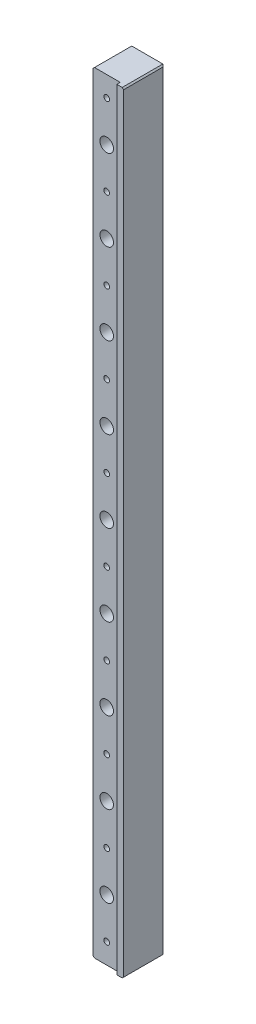
SolidWorks part; units mm, degrees
material "Q235-A"
ref_plane "Front/Back" through (0, 0, 0) normal (0, 0, 1) x (1, 0, 0)
ref_plane "Top/Bottom" through (0, 0, 0) normal (0, 1, 0) x (1, 0, 0)
ref_plane "Right/Left" through (0, 0, 0) normal (1, 0, 0) x (0, 0, -1)
sketch "Sketch1" plane through (0, 0, 0) normal (0, 0, 1) x (1, 0, 0)
  line L0 (-12.5, -285) -> (12.5, 285) construction
  line L1 (-12.5, 285) -> (12.5, 285)
  line L2 (-12.5, 285) -> (-12.5, -285)
  line L3 (-12.5, -285) -> (12.5, -285)
  line L4 (12.5, 285) -> (12.5, -285)
  point P4 (0, 0)
  dimension "D1" = 25
  dimension "D2" = 570
extrude "Extrude1" add sketch "Sketch1" along normal mid plane 30
chamfer "Chamfer1" distance 1 angle 45 4 edges at (12.5, 285, 0) (-12.5, 285, 0) (12.5, -285, 0) (-12.5, -285, 0)
sketch "草图1" plane through (0, 0, 15) normal (0, 0, 1) x (1, 0, 0)
  line L0 (-11.5, -285) -> (11.5, -285) construction
  line L3 (-12.5, 285) -> (7.5, 285)
  line L6 (0, 285) -> (0, -286.2731) construction
  line L7 (11.5, 285) -> (-11.5, 285) construction
  line L9 (-12.5, 285) -> (-12.5, -285)
  line L10 (-12.5, -285) -> (7.5, -285)
  line L11 (7.5, 285) -> (7.5, -285)
  line L12 (12.5, -284) -> (12.5, 284) construction
  line L13 (11.5, 285) -> (-11.5, 285) construction
  line L14 (-12.5, 284) -> (-12.5, -284) construction
  dimension "D1" = 5
extrude "Cut-Extrude1" cut sketch "草图1" against normal blind 2.5
chamfer "Chamfer2" distance 1 angle 45 2 edges at (12.5, 0, -15) (-12.5, 0, -15)
hole_wizard "M5 Tapped Hole1" positions "Sketch2" profile "Sketch3" tap size "M5" standard "GB"
sketch "Sketch2" plane through (0, 0, 12.5) normal (0, 0, 1) x (1, 0, 0)
  point P0 (-2.5, -270)
  point P5 (-2.5, -210)
  point P8 (-2.5, -150)
  point P11 (-2.5, -90)
  point P14 (-2.5, -30)
  point P17 (-2.5, 30)
  point P22 (-2.5, 90)
  point P25 (-2.5, 150)
  point P28 (-2.5, 210)
  point P31 (-2.5, 270)
sketch "Sketch3" plane through (-2.5, -270, 12.5) normal (1, 0, 0) x (0, -1, 0)
  line L0 (0, 0) -> (0, 15.2618)
  line L1 (0, 15.2618) -> (2.1, 14)
  line L2 (2.1, 14) -> (2.1, 0)
  line L5 (2.1, 0) -> (0, 0)
  line L10 (0, 15.2618) -> (-2.1, 14) construction
  line L11 (0, -6.35) -> (0, 107.95) construction
  dimension "螺纹孔钻头直径" = 4.2
  dimension "螺纹孔钻头深度" = 14
  dimension "导头角度" = 118
cosmetic thread "Cosmetic thread 1" parameters "D1"=10, "D2"=5
cosmetic thread "Cosmetic thread 2" parameters "D1"=10, "D2"=5
cosmetic thread "Cosmetic thread 3" parameters "D1"=10, "D2"=5
cosmetic thread "Cosmetic thread 4" parameters "D1"=10, "D2"=5
cosmetic thread "Cosmetic thread 5" parameters "D1"=10, "D2"=5
cosmetic thread "Cosmetic thread 6" parameters "D1"=10, "D2"=5
cosmetic thread "Cosmetic thread 7" parameters "D1"=10, "D2"=5
cosmetic thread "Cosmetic thread 8" parameters "D1"=10, "D2"=5
cosmetic thread "Cosmetic thread 9" parameters "D1"=10, "D2"=5
cosmetic thread "Cosmetic thread 10" parameters "D1"=10, "D2"=5
hole_wizard "Hole size (per socket head cap screw type)1" positions "Sketch4" profile "Sketch5" counterbore size "M5" standard "GB" end condition through all
sketch "Sketch4" plane through (0, 0, 12.5) normal (0, 0, 1) x (1, 0, 0)
  line L0 (-2.5, 270) -> (-2.5, 210)
  point P0 (-2.5, 240)
sketch "Sketch5" plane through (-2.5, 240, 12.5) normal (1, 0, 0) x (0, -1, 0)
  line L0 (0, 0) -> (0, 27.5)
  line L1 (0, 27.5) -> (2.75, 27.5)
  line L3 (2.75, 27.5) -> (2.75, 8)
  line L4 (2.75, 8) -> (5, 8)
  line L5 (5, 8) -> (5, 0)
  line L7 (5, 0) -> (0, 0)
  line L11 (0, -6.35) -> (0, 107.95) construction
  dimension "通孔孔直径" = 5.5
  dimension "通孔孔深度" = 27.5
  dimension "柱形沉头孔直径" = 10
  dimension "柱形沉头孔深度" = 8
pattern_linear "LPattern1" count 9 spacing 60 along (0, -1, 0) of "Hole size (per socket head cap screw type)1"
